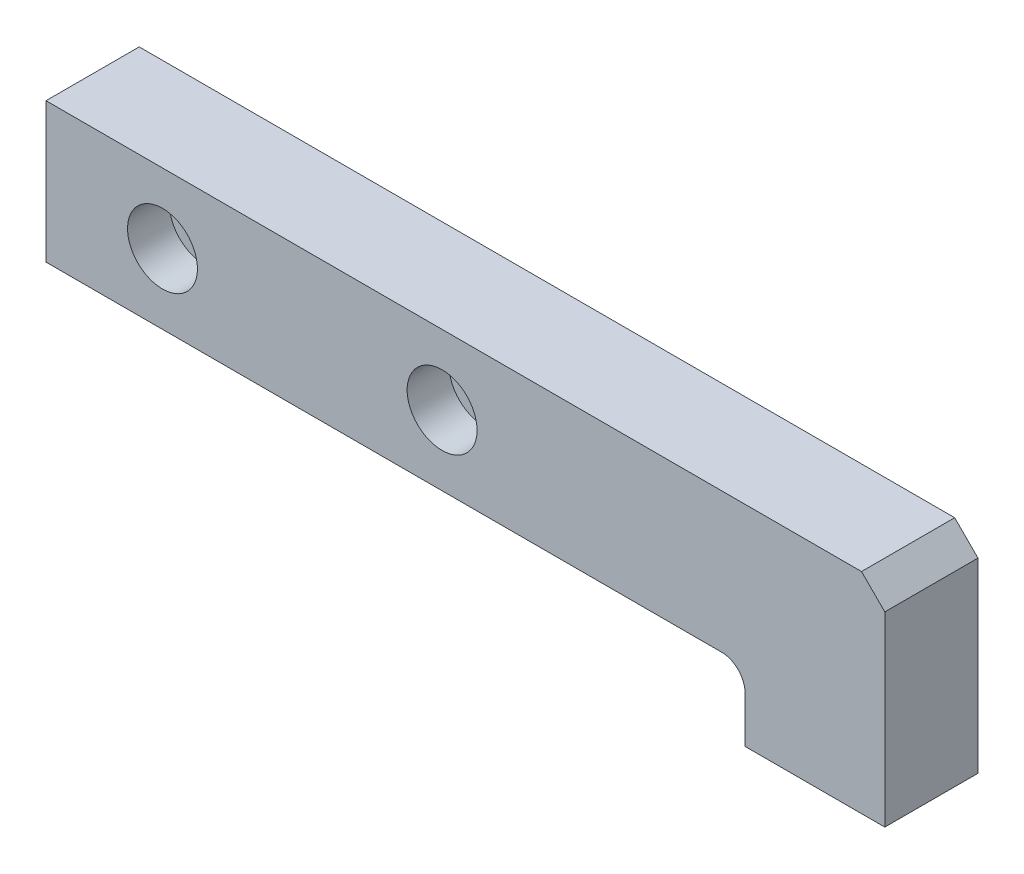
SolidWorks part; units mm, degrees
material "Q235A"
ref_plane "前视基准面" through (0, 0, 0) normal (0, 0, 1) x (1, 0, 0)
ref_plane "上视基准面" through (0, 0, 0) normal (0, 1, 0) x (1, 0, 0)
ref_plane "右视基准面" through (0, 0, 0) normal (1, 0, 0) x (0, 0, -1)
sketch "草图1" plane through (0, 0, 0) normal (0, 0, 1) x (1, 0, 0)
  line L1 (-90, 15) -> (90, 15)
  line L2 (-90, 15) -> (-90, -15)
  line L3 (-90, -15) -> (90, -15)
  line L4 (90, 15) -> (90, -15)
  line L5 (-90, 15) -> (90, -15) construction
  line L6 (-90, -15) -> (90, 15) construction
  point P0 (0, 0)
  dimension "D1" = 180
  dimension "400" = 30
extrude "凸台-拉伸1" add sketch "草图1" along normal blind 20
hole_wizard "打孔尺寸(%根据)内六角圆柱头螺钉的类型1" positions "草图2" profile "草图3" counterbore size "M8" standard "GB" end condition through all
sketch "草图2" plane through (0, 0, 20) normal (0, 0, 1) x (1, 0, 0)
  line L0 (-65, 0) -> (-5, 0) construction
  line L2 (-90, 0) -> (-65, 0) construction
  line L3 (-90, 15) -> (-90, -15) construction
  point P0 (-65, 0)
  point P2 (-5, 0)
  dimension "D1" = 60
  dimension "D2" = 25
sketch "草图3" plane through (-65, 0, 20) normal (1, 0, 0) x (0, -1, 0)
  line L0 (0, 0) -> (0, 20)
  line L1 (0, 20) -> (4.5, 20)
  line L3 (4.5, 20) -> (4.5, 9)
  line L4 (4.5, 9) -> (7.5, 9)
  line L5 (7.5, 9) -> (7.5, 0)
  line L7 (7.5, 0) -> (0, 0)
  line L11 (0, -6.35) -> (0, 107.95) construction
  dimension "通孔孔直径" = 9
  dimension "通孔孔深度" = 20
  dimension "柱形沉头孔直径" = 15
  dimension "柱形沉头孔深度" = 9
sketch "草图4" plane through (0, 0, 20) normal (0, 0, 1) x (1, 0, 0)
  line L0 (90, -15) -> (90, -30)
  line L1 (90, -30) -> (60, -30)
  line L2 (60, -30) -> (60, -15)
  line L3 (-90, -15) -> (90, -15) construction
  line L4 (90, 15) -> (-90, 15) construction
  line L5 (60, -15) -> (90, -15)
  dimension "D1" = 30
  dimension "D2" = 45
extrude "凸台-拉伸2" add sketch "草图4" against normal up to surface (20 mm away) contours L0 L1 L2 L5 up to face at (-60.5, 0, 0)
fillet "圆角1" radius 5 1 edges at (60, -15, 10)
chamfer "倒角1" distance 5 angle 45 1 edges at (90, 15, 10)
hole_wizard "M8 螺纹孔2" positions "草图5" profile "草图6" tap size "M8" standard "GB"
sketch "草图5" plane through (0, -30, 0) normal (0, -1, 0) x (-1, 0, 0)
  line L0 (-75, 0) -> (-75, -10) construction
  line L1 (-60, 0) -> (-90, 0) construction
  line L2 (-75, -10) -> (-90, -10) construction
  line L3 (-90, 0) -> (-90, -20) construction
  point P0 (-75, -10)
sketch "草图6" plane through (75, -30, 10) normal (1, 0, 0) x (0, 0, -1)
  line L0 (0, 0) -> (0, 21.7929)
  line L1 (0, 21.7929) -> (3.4, 19.75)
  line L2 (3.4, 19.75) -> (3.4, 0)
  line L5 (3.4, 0) -> (0, 0)
  line L10 (0, 21.7929) -> (-3.4, 19.75) construction
  line L11 (0, -6.35) -> (0, 107.95) construction
  dimension "螺纹孔钻头直径" = 6.8
  dimension "螺纹孔钻头深度" = 19.75
  dimension "导头角度" = 118
cosmetic thread "孔螺蚊线1" parameters "D1"=16, "D2"=8
